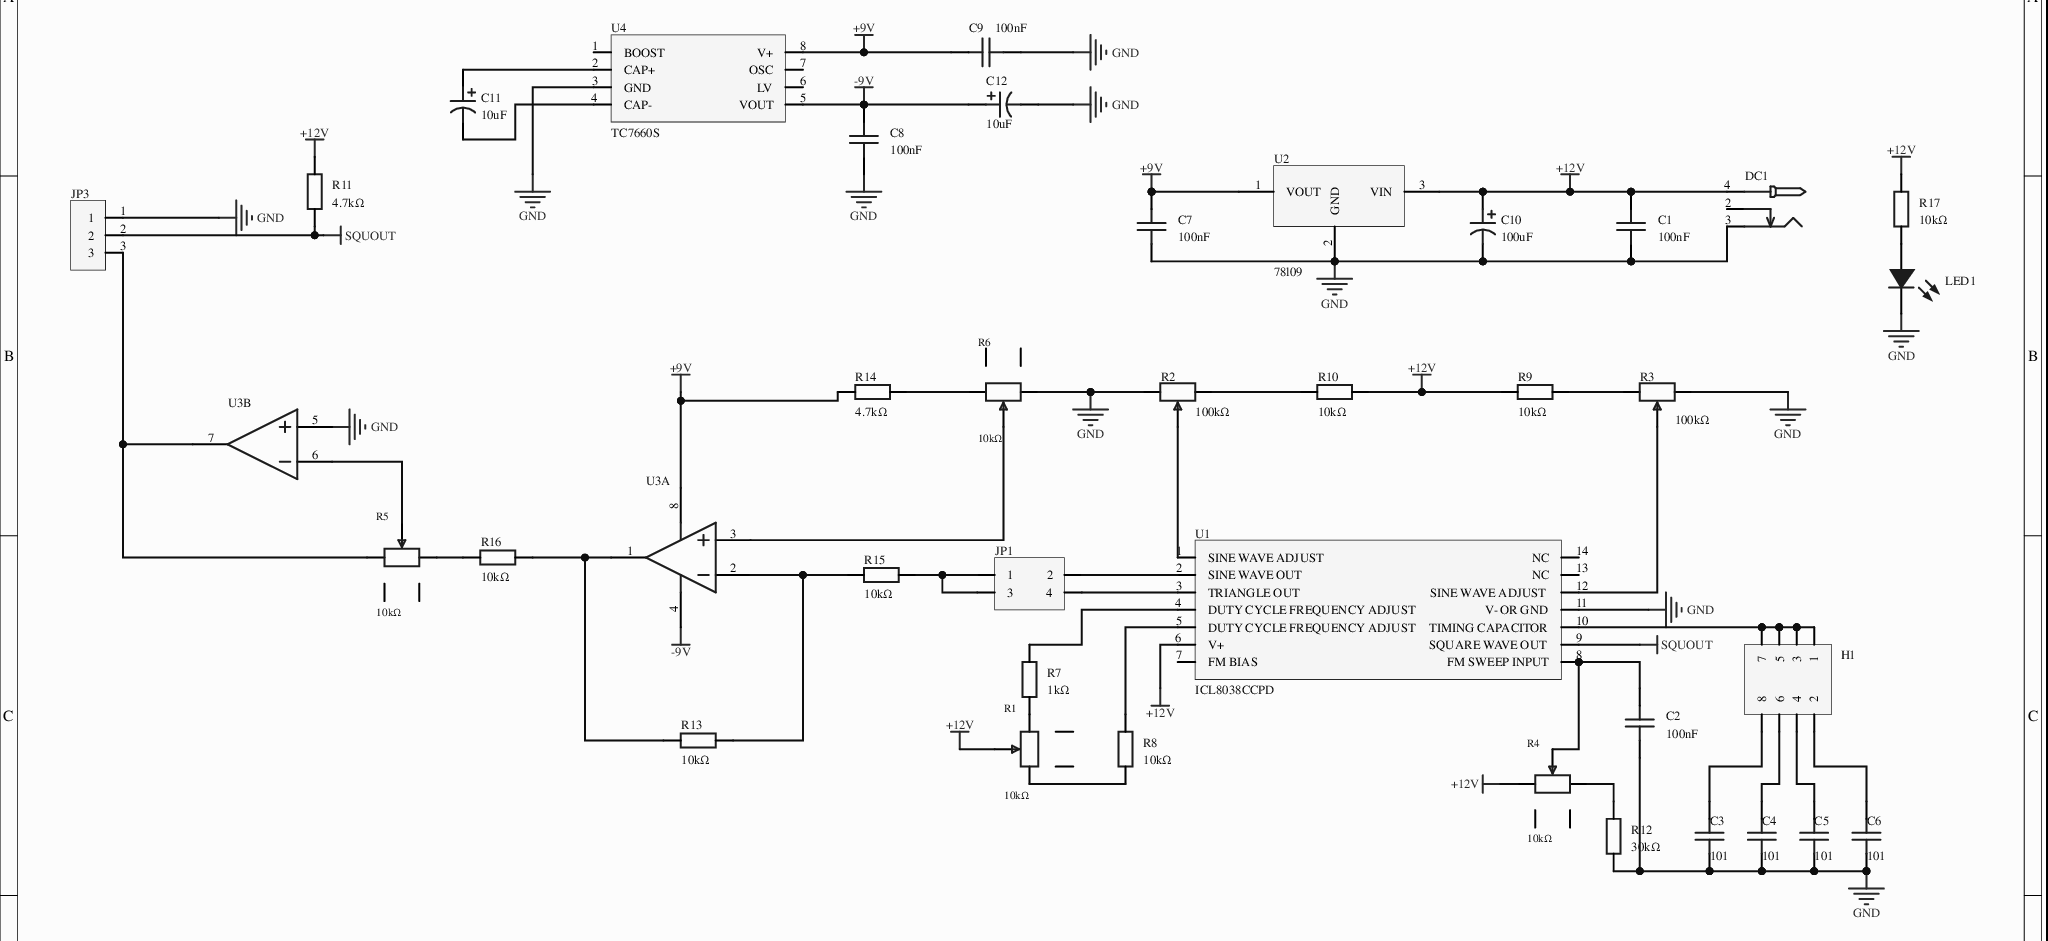
[diagram p0: MISC49930-3.schdoc]
# Altium project MISC49930-2.PrjPcb
1 sheet, 38 parts. Net scope: global (net labels, ports and power ports of the same name join across sheets).
Board file: MISC49930.pcbdoc

## Sheet MISC49930-3.schdoc
size 297 x 209 mm; Version: V1.0; @Project Name: MISC49930; @Update Date: 2026-09-21; @Create Date: 2026-09-21; @Board Name: MISC49930; @Create Time: 22:26:39; @Page Count: 1; @Page No: 1; @Schematic Name: MISC49930; @Update Time: 22:26:39; Size: A4

### Parts
C1  100nF  [CAP-TH_L5.1-W3.2-P5.08-D0.50]
C2  100nF  [CAP-TH_L5.1-W3.2-P5.08-D0.50]
C3  101  [CAP-TH_L5.1-W3.2-P5.08-D0.50]
C4  101  [CAP-TH_L5.1-W3.2-P5.08-D0.50]
C5  101  [CAP-TH_L5.1-W3.2-P5.08-D0.50]
C6  101  [CAP-TH_L5.1-W3.2-P5.08-D0.50]
C7  100nF  [CAP-TH_L5.1-W3.2-P5.08-D0.50]
C8  100nF  [CAP-TH_L5.1-W3.2-P5.08-D0.50]
C9  100nF  [CAP-TH_L5.1-W3.2-P5.08-D0.50]
C10  100uF  [CAP-TH_BD6.3-P2.5-D0.6-FD-RYHG35V100UF]
C11  10uF  [CAP-TH_BD5.0-P2.00-D0.8-FD-10UF50VC110GL]
C12  10uF  [CAP-TH_BD5.0-P2.00-D0.8-FD-10UF50VC110GL]
DC1  (no value)  [DC-2.0]
H1  (no value)  [HDR-TH_8P-P2.54-V-F-R2-C4-S2.54-1]
JP1  (no value)  [HDR-TH_4P-P2.54-V-F-R2-C2-S2.54]
JP3  (no value)  [CONN-TH_3P-P5.00_KF301-5.0-3P]
LED1  (no value)  [LED_TH-3mm]
R1  10kΩ  [RES-ADJ-TH_R09512N0-FB15A7.0-B103-005]
R2  100kΩ  [RES-ADJ-SMD_RM065-V1]
R3  100kΩ  [RES-ADJ-SMD_RM065-V1]
R4  10kΩ  [RES-ADJ-TH_R09512N0-FB15A7.0-B103-005]
R5  10kΩ  [RES-ADJ-TH_R09512N0-FB15A7.0-B103-005]
R6  10kΩ  [RES-ADJ-TH_R09512N0-FB15A7.0-B103-005]
R7  1kΩ  [Res_1/4W]
R8  10kΩ  [Res_1/4W]
R9  10kΩ  [Res_1/4W]
R10  10kΩ  [Res_1/4W]
R11  4.7kΩ  [Res_1/4W]
R12  30kΩ  [Res_1/4W]
R13  10kΩ  [Res_1/4W]
R14  4.7kΩ  [Res_1/4W]
R15  10kΩ  [Res_1/4W]
R16  10kΩ  [Res_1/4W]
R17  10kΩ  [Res_1/4W]
U1  ICL8038CCPD  [PDIP-14_L19.2-W6.6-P2.54-LS7.6-BL]
U2  78l09  [TO-92-3_L4.5-W3.5-P1.27-L]
U3  (no value)  [DIP-8_L9.3-W6.4-P2.54-LS7.6-TL]  (parts A,B of 2)
U4  TC7660S  [DIP-8_L10.0-W6.5-P2.54-LS7.6-BL]

### Nets
+9V: C7.2 C9.2 R14.1 U2.1(VOUT) U3.8(VCC+) U4.8(V+)
+12V: C1.2 C10.1 DC1.4 R1.2 R4.3 R9.1 R10.2 R11.2 R17.2 U1.6(V+) U2.3(VIN)
-9V: C8.2 C12.1 U3.4(VCC-) U4.5(VOUT)
GND: C1.1 C2.1 C3.1 C4.1 C5.1 C6.1 C7.1 C8.1 C9.1 C10.2 C12.2 DC1.3 JP3.1 LED1.2(A) R2.3 R3.1 R6.3 R12.1 U1.11(V-_OR_GND) U2.2(GND) U3.5(2IN+) U4.3(GND)
SQUOUT: JP3.2 R11.1 U1.9(SQUARE_WAVE_OUT)
NetC2_2: C2.2 R4.2 U1.8(FM_SWEEP_INPUT)
NetC3_2: C3.2 H1.8
NetC4_2: C4.2 H1.6
NetC5_2: C5.2 H1.4
NetC6_2: C6.2 H1.2
NetC11_1: C11.1 U4.2(CAP+)
NetC11_2: C11.2 U4.4(CAP-)
NetH1_1: H1.1 H1.3 H1.5 H1.7 U1.10(TIMING_CAPACITOR)
NetJP1_1: JP1.1 JP1.3 R15.2
NetJP1_2: JP1.2 U1.2(SINE_WAVE_OUT)
NetJP1_4: JP1.4 U1.3(TRIANGLE_OUT)
NetJP3_3: JP3.3 R5.3 U3.7(2OUT)
NetLED1_1: LED1.1(C) R17.1
NetR1_1: R1.1 R7.1
NetR1_3: R1.3 R8.1
NetR2_1: R2.1 R10.1
NetR2_2: R2.2 U1.1(SINE_WAVE_ADJUST)
NetR3_2: R3.2 U1.12(SINE_WAVE_ADJUST)
NetR3_3: R3.3 R9.2
NetR4_1: R4.1 R12.2
NetR5_1: R5.1 R16.1
NetR5_2: R5.2 U3.6(2IN-)
NetR6_1: R6.1 R14.2
NetR6_2: R6.2 U3.3(1IN+)
NetR7_2: R7.2 U1.4(DUTY_CYCLE_FREQUENCY_ADJUST)
NetR8_2: R8.2 U1.5(DUTY_CYCLE_FREQUENCY_ADJUST)
NetR13_1: R13.1 R16.2 U3.1(1OUT)
NetR13_2: R13.2 R15.1 U3.2(1IN-)

Not connected (* = marked no-connect by the designer): DC1 2*; R1 4* 5*; R4 4* 5*; R5 4* 5*; R6 4* 5*; U1 7(FM_BIAS)* 13(NC)* 14(NC)*; U4 1(BOOST)* 6(LV)* 7(OSC)*

### Library data of the parts
C1-C9 = C323C104K5R5TA7301: Capacitance:100nF; tolerance:±10%; rated voltage:50V; temperature coefficient:X7R;; Manufacturer: KEMET(基美); 3D Model: 5e578892460b443ea6286c5f4e214fbb0819f05c4eef4c71ace90d822a990e87; 3D Model Transform: 219.6846,125.5903,0,0,0,0,0,0,-196.85; Tolerance: ±10%; Voltage Rating: 50V; Temperature Coefficient: X7R; Pin Spacing: 5.08mm; AddInBom: yes; Symbol: C323C104K5R5TA7301; Device: C323C104K5R5TA7301; LCSC Part Name: 100nF ±10% 50V; Manufacturer Part: C323C104K5R5TA7301; Supplier Footprint: 插件,P=5.08mm; JLCPCB Part Class: Extended Part; Datasheet: https://item.szlcsc.com/datasheet/C323C104K5R5TA7301/194969.html; Supplier: LCSC; FootprintName: CAP-TH_L5.1-W3.2-P5.08-D0.50; ConvertToPcb: yes; ModelName: CAP-TH_L5.1-W3.2-P5.08-D0.50
  C1 C2 C7-C9: Supplier Part: C183565; Value: 100nF
  C3-C6: Value: 101
C10 = RYHG35V100UF6*8: Capacitance:100uF; rated voltage:35V; ripple current:2.25A@100kHz; equivalent series resistance (ESR):38mΩ@100kHz; type:polymer;; Manufacturer: HONOR(荣誉); 3D Model: 12e6233a919142bb8336abc71a80483c0819f05c4eef4c71ace90d822a990e87; 3D Model Transform: 249.99647,248.42,0,0,0,0,0,0,-196.85; Voltage Rating: 35V; Lifetime: 2000hrs@105℃; Polarity type: Polarized; AddInBom: yes; Symbol: RYHG35V100UF6*8; Device: RYHG35V100UF6*8; LCSC Part Name: 100uF 35V; Supplier Part: C48970442; Manufacturer Part: RYHG35V100UF6*8; Supplier Footprint: 插件,D6.3xL8mm; JLCPCB Part Class: Extended Part; Datasheet: https://item.szlcsc.com/datasheet/RYHG35V100UF6*8/51295386.html; Supplier: LCSC; Value: 100uF; Ripple Current: 2.25A@100kHz; Equivalent Series Resistance(ESR): 38mΩ@100kHz; Type: Polymer; Diameter: 6.3mm; Height - Seated (Max): 8mm; FootprintName: CAP-TH_BD6.3-P2.5-D0.6-FD-RYHG35V100UF; ConvertToPcb: yes; ModelName: CAP-TH_BD6.3-P2.5-D0.6-FD-RYHG35V100UF
C11 C12 = 10UF50VC110GL: Capacitance:10uF; tolerance:±20%; rated voltage:50V; ripple current:120mA@100KHz; equivalent series resistance (ESR):1.6Ω;; Manufacturer: Econd(米朗电子); 3D Model: b35ab6b0460c4c43a629d91cfc2b58780819f05c4eef4c71ace90d822a990e87; 3D Model Transform: 196.85,196.85,0,0,0,0,0,0,-196.85; Tolerance: ±20%; Voltage Rating: 50V; Equivalent Series Resistance(ESR): 1.6Ω; Pin Spacing: 2mm; Lifetime: 5000hrs@105℃; AddInBom: yes; Symbol: 10UF50VC110GL; Device: 10UF50VC110GL; LCSC Part Name: 10uF ±20% 50V; Supplier Part: C46867109; Manufacturer Part: 10UF50VC110GL; Supplier Footprint: 插件,D5xL11mm; JLCPCB Part Class: Extended Part; Datasheet: https://item.szlcsc.com/datasheet/10UF50VC110GL/49031974.html; Supplier: LCSC; Value: 10uF; Ripple Current: 120mA@100KHz; Diameter: 5mm; Height - Seated (Max): 11mm; Operating Temperature: -40℃~+105℃; FootprintName: CAP-TH_BD5.0-P2.00-D0.8-FD-10UF50VC110GL; ConvertToPcb: yes; ModelName: CAP-TH_BD5.0-P2.00-D0.8-FD-10UF50VC110GL
DC1 = DC-005_2.0: Symbol: DC power connector; 3D Model: f5f20b8a2308479b936ba3c2698865bb0819f05c4eef4c71ace90d822a990e87; 3D Model Transform: 372.05,551.18,582.68,90,0,0,137.8,0,-149.61; ConvertToPcb: yes; ModelName: DC-IN-TH_DC-5520-1; Device: DC-005_2.0; Supplier Footprint: 插件; FootprintName: DC-2.0; AddInBom: yes
H1 = HDR-F_2.54_2x4: Symbol: HDR-F-2.54_2x4; 3D Model: 64729f32a5874cf59655d275a66f10500819f05c4eef4c71ace90d822a990e87; 3D Model Transform: 399.999,200,0,0,0,0,0,0,-118.11; ConvertToPcb: yes; ModelName: HDR2.54-F-LI-2X4P; Device: HDR-F_2.54_2x4; Supplier Part: C92271; Supplier Footprint: 插件; FootprintName: HDR-TH_8P-P2.54-V-F-R2-C4-S2.54-1; AddInBom: yes
JP1 = HDR-F_2.54_2x2: Symbol: HDR-F-2.54_2x2; 3D Model: 870c884146ee4765973edc845f10b7af0819f05c4eef4c71ace90d822a990e87; 3D Model Transform: 215.7476,196.85,0,0,0,0,0,0,-118.11; ConvertToPcb: yes; ModelName: HDR-TH_4P-P2.54-F-LI-2X2P; Device: HDR-F_2.54_2x2; Supplier Part: C92273; Supplier Footprint: 插件; FootprintName: HDR-TH_4P-P2.54-V-F-R2-C2-S2.54; AddInBom: yes
JP3 = HDR-M_2.54_1x3P: 3D Model: bb473b6d38ff42a99216a4fcdbdcc4cb0819f05c4eef4c71ace90d822a990e87; 3D Model Transform: 300.03877,100,0,0,0,0,0,0,-118.11; AddInBom: yes; ModelName: HDR-TH_3P-P2.54-M-LI-1X3P; Symbol: HDR-M_2.54_1x3P; Device: HDR-M_2.54_1x3P; Supplier Part: C2937625; Supplier Footprint: 插件; ConvertToPcb: yes; FootprintName: CONN-TH_3P-P5.00_KF301-5.0-3P
LED1 = LED_TH-R_3mm: 3D Model: a497c992633541038a38947cdc58012f0819f05c4eef4c71ace90d822a990e87; 3D Model Transform: 141.274,153.327,0,0,0,0,-5.984,0,-137.795; ConvertToPcb: yes; ModelName: LED-TH-3mm_R; Symbol: LED_TH-R; Device: LED_TH-R_3mm; Supplier Footprint: 插件; FootprintName: LED_TH-3mm; AddInBom: yes
R1 R4-R6 = R09592N0-AE4.5C3.0-B104-0007: Resistance:100kΩ; tolerance:±10%; power:50mW;; Manufacturer: CTR(长泰尔电子); 3D Model: af2b700c287243e8ae02a32afb53b47a0819f05c4eef4c71ace90d822a990e87; 3D Model Transform: 464.669,486.2195,0,0,0,0,0,86.616,-137.795; Tolerance: ±10%; Voltage Rating: 10V; Power(Watts): 50mW; AddInBom: yes; Symbol: R09592N0-AE4.5C3.0-B104-0007; Device: R09592N0-AE4.5C3.0-B104-0007; Value: 10kΩ; LCSC Part Name: 电位器; Manufacturer Part: R09592N0-AE4.5C3.0-B104-0007; Supplier Footprint: 插件; JLCPCB Part Class: Extended Part; Datasheet: https://item.szlcsc.com/datasheet/R09592N0-AE4.5C3.0-B104-0007/19388962.html; Supplier: LCSC; FootprintName: RES-ADJ-TH_R09512N0-FB15A7.0-B103-005; ConvertToPcb: yes; ModelName: RES-ADJ-TH_R09512N0-FB15A7.0-B103-005
R2 R3 = RM065-103(10K): Resistance:10kΩ; tolerance:±25%; power:100mW;; Manufacturer: BOCHEN(博晨); 3D Model: c816c2b7942147f5a832150e8ef6960c0819f05c4eef4c71ace90d822a990e87; 3D Model Transform: 255.905,283.464,0,0,0,0,0.025,-3.937,-157.48; Tolerance: ±25%; Voltage Rating: 50V; Power(Watts): 100mW; AddInBom: yes; Symbol: RM065-103(10K); Device: RM065-103(10K); Value: 100kΩ; LCSC Part Name: 10kΩ ±25%; Manufacturer Part: RM065-103(10K); Supplier Footprint: 插件,7.3x6.4mm; JLCPCB Part Class: Extended Part; Datasheet: https://item.szlcsc.com/datasheet/RM065-103(10K)/5896379.html; Supplier: LCSC; FootprintName: RES-ADJ-SMD_RM065-V1; ConvertToPcb: yes; ModelName: RES-ADJ-SMD_RM065-V1
R7-R17 = Res_AXIAL-1/8W: Symbol: Resistor; 3D Model: b2b5ae7ae4c642178fe0039925c86a3f0819f05c4eef4c71ace90d822a990e87; 3D Model Transform: 282.86,66.88,253.09,0,0,0,0,0,-191; ConvertToPcb: yes; ModelName: RES-TH_BD1.8-L3.2-P7.20-D0.4; Device: Res_AXIAL-1/8W; Supplier Footprint: 轴向引线; AddInBom: yes; FootprintName: Res_1/4W
  R7: Value: 1kΩ
  R8-R10 R13 R15-R17: Value: 10kΩ
  R11 R14: Value: 4.7kΩ
  R12: Value: 30kΩ
U1 = ICL8038CCPD_C5274778: Interface type:-; max output frequency:-; output channels:4;; Manufacturer: Sungine(双竞集成); 3D Model: 08aeb3774ab0450ba412f07c9830bd710819f05c4eef4c71ace90d822a990e87; 3D Model Transform: 755.904,309.842,0,0,0,0,0,0,-129.921; Number of Outputs: 4; Clock/Oscillator: External; Output: TTL; AddInBom: yes; Symbol: ICL8038CCPD_C5274778; Device: ICL8038CCPD_C5274778; LCSC Part Name: ICL8038CCPD 停产; Supplier Part: C5274778; Manufacturer Part: ICL8038CCPD; Supplier Footprint: DIP-14; JLCPCB Part Class: Extended Part; Datasheet: https://item.szlcsc.com/datasheet/ICL8038CCPD/6005916.html; Supplier: LCSC; Interface: -; Output Frequency(Max): -; Voltage - Supply: -; Operating Temperature: 0℃~+70℃; Period Jitter: -; Cycle-to-Cycle Jitter: -; Phase Jitter: -; Phase Offset: -; Input: -; Features: -; FootprintName: PDIP-14_L19.2-W6.6-P2.54-LS7.6-BL; ConvertToPcb: yes; ModelName: PDIP-14_L19.2-W6.6-P2.54-LS7.6-BL
U2 = 78l09: Symbol: 78xx; BOM名称: Linear regulator IC; AddInBom: yes; Device: 78l09; ConvertToPcb: yes
U3 = TL082: Relevance: []; 3D Model: 4f1f5228684a45afaa7af8cce46001de775e0ad868094fe081de71bc42b56d73; 3D Model Transform: 236.97,190.17000000000002,64.01,0,0,0,108.27,72.5,0; AddInBom: yes; ModelName: SOP-8_L4.9-W3.9-H1.5-LS6.0-P1.27; Symbol: TL082; Device: TL082; ConvertToPcb: yes; FootprintName: DIP-8_L9.3-W6.4-P2.54-LS7.6-TL
U4 = TC7660S: Manufacturer: null; AddInBom: yes; Symbol: TC7660S; Device: TC7660S; link: https://item.szlcsc.com/241216.html; Supplier Part: null; Supplier: null; 3DModel: DIP-8_L10.0-W6.5-P2.54-LS7.6-BL; JLCPCB Part Class: Extended Part; FootprintName: DIP-8_L10.0-W6.5-P2.54-LS7.6-BL; ConvertToPcb: yes